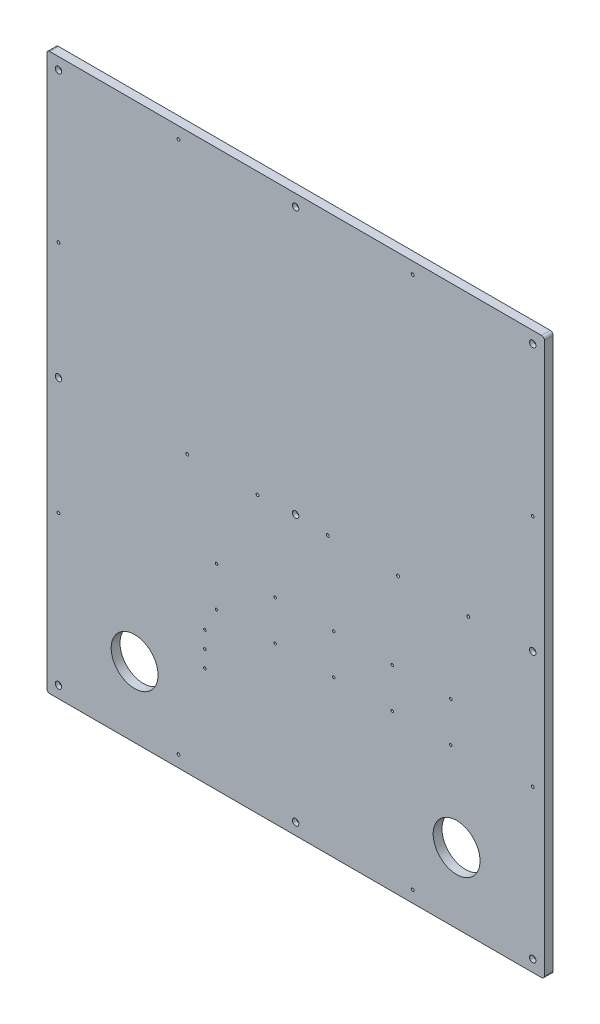
from build123d import *

# Parameters (mm, degrees)
SKETCH_1_W                = 850
SKETCH_1_H                = 950
EXTRUDE_1_DEPTH           = 15
FILLET_1_R                = 5
HOLE_WIZARD_M5_1_D        = 4.2
PATTERN_LINEAR_1_COUNT    = 5
PATTERN_LINEAR_1_PITCH    = 100
HOLE_WIZARD_M6_1_D        = 5
CUT_EXTRUDE_1_REACH       = 639.554
SKETCH_6_R                = 40
HOLE_WIZARD_M5_2_D        = 4.2
HOLE_WIZARD_1_D           = 6.6
HOLE_WIZARD_1_CBORE_D     = 11
HOLE_WIZARD_1_CBORE_DEPTH = 6.8
HOLE_WIZARD_M6_2_D        = 5


with BuildPart() as part:
    # 草图1 → 凸台-拉伸1 (new body)
    with BuildSketch(Plane.XY):
        Rectangle(SKETCH_1_W, SKETCH_1_H)
    extrude(amount=EXTRUDE_1_DEPTH)

    # 圆角1
    fillet_1_edges = [part.edges().sort_by_distance(p)[0] for p in [
        (-425, 475, 7.5),
        (425, 475, 7.5),
        (425, -475, 7.5),
        (-425, -475, 7.5),
    ]]
    fillet(fillet_1_edges, radius=FILLET_1_R)

    # M5 螺纹孔1 (through all)
    with Locations(Plane.XY.offset(15)):
        with Locations((265, -140.199999647), (265, -208.199999647)):
            hole_wizard_m5_1 = Hole(HOLE_WIZARD_M5_1_D / 2)

    # 阵列(线性)1: M5 螺纹孔1 ×5
    with Locations(*[(-i * PATTERN_LINEAR_1_PITCH, 0, 0) for i in range(1, PATTERN_LINEAR_1_COUNT)]):
        add(hole_wizard_m5_1, mode=Mode.SUBTRACT)

    # M6 螺纹孔1 (through all)
    with Locations(Plane.XY.offset(15)):
        with Locations((-185, -3.399999647), (-65, -3.399999647), (55, -3.399999647), (175, -3.399999647), (295, -3.399999647)):
            Hole(HOLE_WIZARD_M6_1_D / 2)

    # 草图6 → 切除-拉伸1 (cut, up to next)
    with BuildSketch(Plane.XY.offset(15), mode=Mode.PRIVATE) as cut_extrude_1_sk1:
        with Locations((-275, -355)):
            Circle(SKETCH_6_R)
    cut_extrude_1_tool1 = extrude(cut_extrude_1_sk1.sketch, amount=-CUT_EXTRUDE_1_REACH, mode=Mode.PRIVATE) & part.part
    # 草图6 → 切除-拉伸1 (cut, up to next)
    with BuildSketch(Plane.XY.offset(15), mode=Mode.PRIVATE) as cut_extrude_1_sk2:
        with Locations((275, -355)):
            Circle(SKETCH_6_R)
    cut_extrude_1_tool2 = extrude(cut_extrude_1_sk2.sketch, amount=-CUT_EXTRUDE_1_REACH, mode=Mode.PRIVATE) & part.part
    add(cut_extrude_1_tool1.solids().sort_by_distance((-275, -355, 15))[0], mode=Mode.SUBTRACT)
    add(cut_extrude_1_tool2.solids().sort_by_distance((275, -355, 15))[0], mode=Mode.SUBTRACT)

    # M5 螺纹孔2 (through all)
    with Locations(Plane.XY.offset(15)):
        with Locations((-155, -248), (-155, -276.5), (-155, -305)):
            Hole(HOLE_WIZARD_M5_2_D / 2)

    # 打孔尺寸(%根据)内六角圆柱头螺钉的类型1 (through all)
    with Locations(Plane.XY.offset(15)):
        with Locations((-405, -455), (0, -455), (405, -455), (0, 0), (-405, 0), (-405, 455), (0, 455), (405, 455), (405, 0)):
            CounterBoreHole(HOLE_WIZARD_1_D / 2, HOLE_WIZARD_1_CBORE_D / 2, HOLE_WIZARD_1_CBORE_DEPTH)

    # M6 螺纹孔2 (through all)
    with Locations(Plane.XY.offset(15)):
        with Locations((-405, 200), (-405, -200), (-200, -455), (200, -455), (405, -200), (405, 200), (200, 455), (-200, 455)):
            Hole(HOLE_WIZARD_M6_2_D / 2)


solid = part.part
